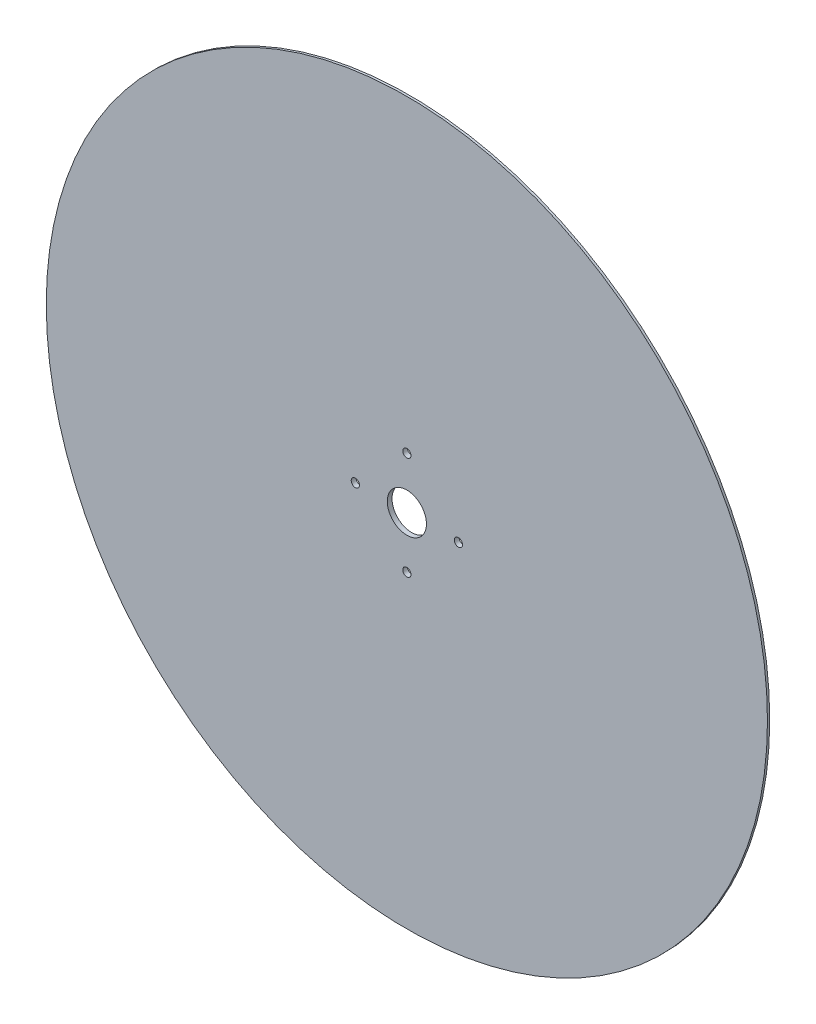
from build123d import *

# Parameters (mm, degrees)
SKETCH_3_R          = 175
EXTRUDE_1_DEPTH     = 1.1
SKETCH_4_R          = 170
EXTRUDE_2_DEPTH     = 1.2
SKETCH_7_R          = 9.5
CUT_EXTRUDE_1_DEPTH = 248.498060598
SKETCH_10_R         = 2
CUT_EXTRUDE_2_DEPTH = 2.3


with BuildPart() as part:
    # 草图3 → 凸台-拉伸1 (new body)
    with BuildSketch(Plane.XY):
        Circle(SKETCH_3_R)
    extrude(amount=EXTRUDE_1_DEPTH)

    # 草图4 → 凸台-拉伸2 (add)
    with BuildSketch(Plane(origin=(0, 0, 0), x_dir=(-1, 0, 0), z_dir=(0, 0, -1))):
        with Locations(Location((0, 0, 0), (0, 0, 180))):
            Circle(SKETCH_4_R)
    extrude(amount=EXTRUDE_2_DEPTH)

    # 草图7 → 切除-拉伸1 (cut, through all)
    with BuildSketch(Plane.XY.offset(1.1)):
        Circle(SKETCH_7_R)
    extrude(amount=-CUT_EXTRUDE_1_DEPTH, mode=Mode.SUBTRACT)

    # 扫描1: sweep along a path in 草图9
    with BuildLine(Plane(origin=(0, 0, 0), x_dir=(-1, 0, 0), z_dir=(0, 0, -1))) as sweep_1_path:
        CenterArc((0, 0), 170, 0, 360)
    # 草图8 → 扫描1 (sweep)
    with BuildSketch(Plane(origin=(0, 0, 0), x_dir=(1, 0, 0), z_dir=(0, 1, 0))):
        Polygon((-175, 0), (-170, 1.2), (-170, 0), align=None)
    sweep(path=sweep_1_path.line)

    # 草图10 → 切除-拉伸2 (cut)
    with BuildSketch(Plane.XY.offset(1.1)):
        with Locations((0, 25)):
            Circle(SKETCH_10_R)
        with Locations((25, 0)):
            Circle(SKETCH_10_R)
        with Locations((0, -25)):
            Circle(SKETCH_10_R)
        with Locations((-25, 0)):
            Circle(SKETCH_10_R)
    extrude(amount=-CUT_EXTRUDE_2_DEPTH, mode=Mode.SUBTRACT)


solid = part.part
